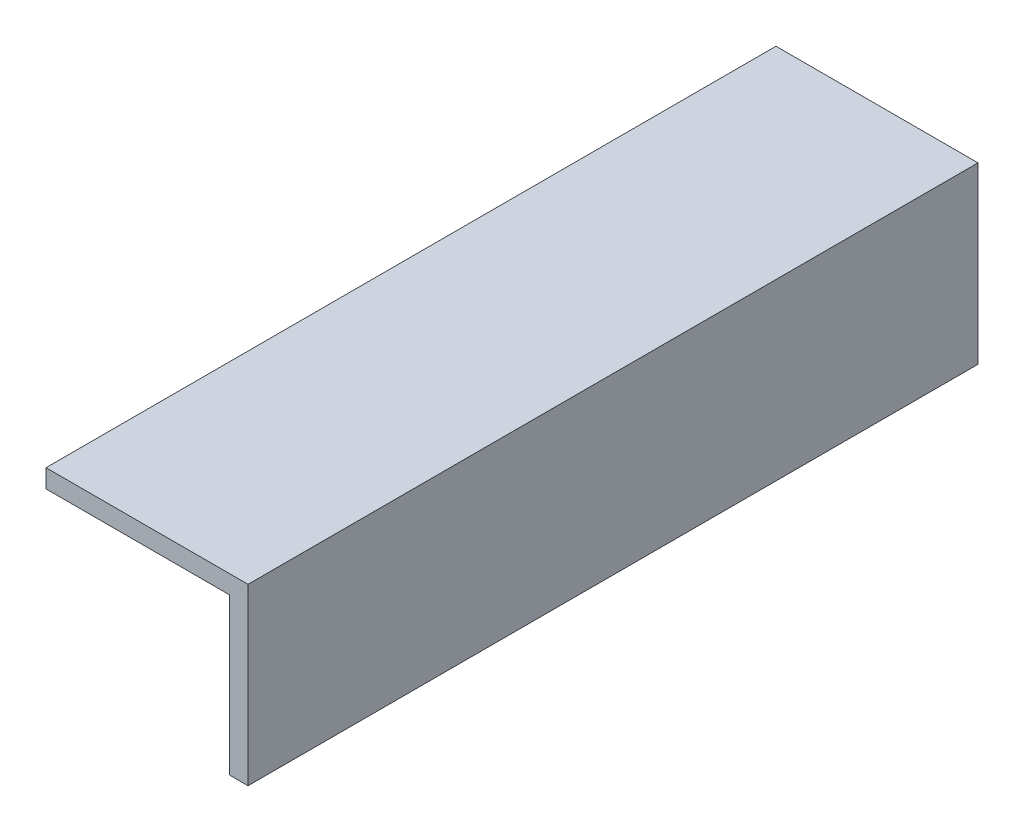
from build123d import *

# Parameters (mm, degrees)
EXTRUDE_1_DEPTH = 300
EXTRUDE_2_DEPTH = 10
EXTRUDE_3_DEPTH = 8
SKETCH_5_W      = 8
SKETCH_5_H      = 318
EXTRUDE_4_DEPTH = 8


with BuildPart() as part:
    # 草图1 → 凸台-拉伸1 (new body)
    with BuildSketch(Plane.XY):
        Polygon((0, 0), (0, 60), (-80, 60), (-80, 68), (8, 68), (8, 0), align=None)
    extrude(amount=EXTRUDE_1_DEPTH)

    # 草图2 → 凸台-拉伸2 (add)
    with BuildSketch(Plane.XY.offset(300)):
        Polygon((0, 0), (8, 0), (8, 68), (-80, 68), (-80, 60), (0, 60), align=None)
    extrude(amount=EXTRUDE_2_DEPTH)

    # 草图4 → 凸台-拉伸3 (add)
    with BuildSketch(Plane(origin=(0, 0, 0), x_dir=(-1, 0, 0), z_dir=(0, 0, -1))):
        Polygon((-8, 0), (0, 0), (0, 60), (80, 60), (80, 68), (-8, 68), align=None)
    extrude(amount=EXTRUDE_3_DEPTH)

    # 草图5 → 凸台-拉伸4 (add)
    with BuildSketch(Plane.XZ):
        with Locations((4, 151)):
            Rectangle(SKETCH_5_W, SKETCH_5_H)
    extrude(amount=EXTRUDE_4_DEPTH)


solid = part.part
